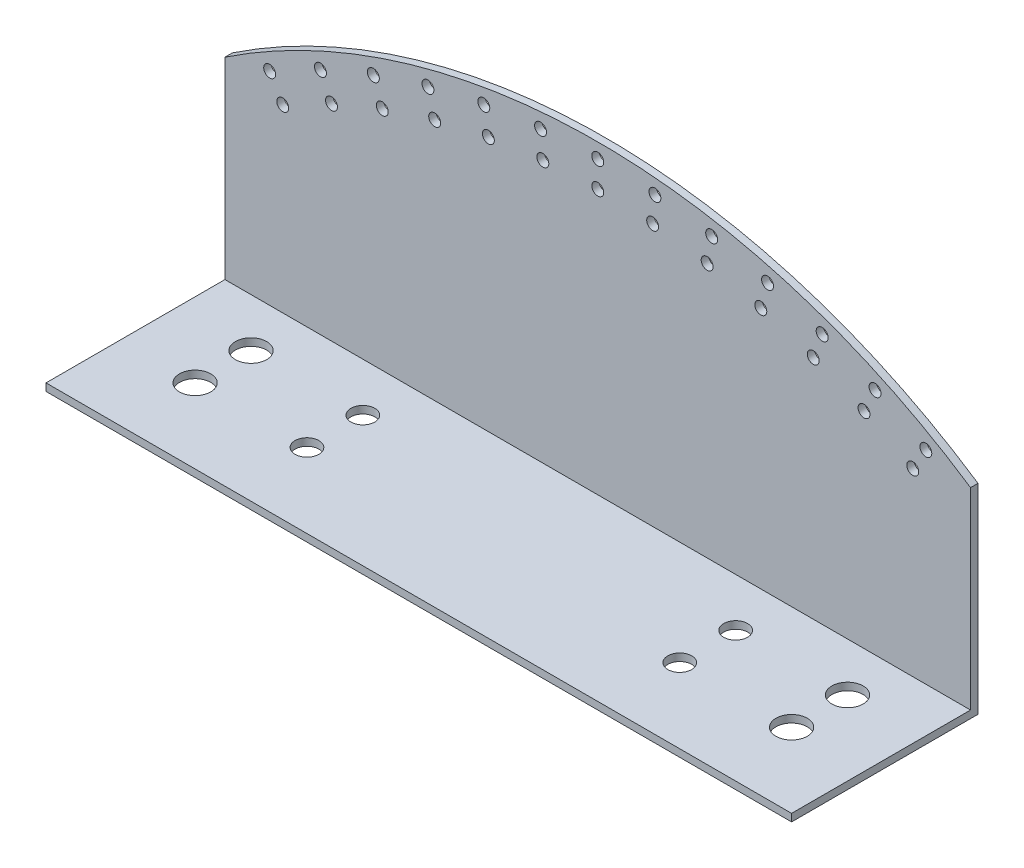
from build123d import *

# Parameters (mm, degrees)
SKETCH_1_R          = 1.6
EXTRUDE_1_DEPTH     = 2
SKETCH_2_W          = 200
SKETCH_2_H          = 2
EXTRUDE_2_DEPTH     = 48
SKETCH_3_R          = 3.2
SKETCH_3_R_2        = 4.2
CUT_EXTRUDE_1_DEPTH = 48


with BuildPart() as part:
    # 草图1 → 凸台-拉伸1 (new body)
    with BuildSketch(Plane.XY):
        with BuildLine():
            Line((1437.273715593, 307.480108419), (1237.273715593, 307.480108419))
            Line((1237.273715593, 307.480108419), (1237.273715593, 361.14640389))
            ThreePointArc((1237.273715593, 361.14640389), (1337.273715593, 391.480108419), (1437.273715593, 361.14640389))
            Line((1437.273715593, 361.14640389), (1437.273715593, 307.480108419))
        make_face()
        with Locations((1337.273715593, 387.480108419)):
            Circle(SKETCH_1_R, mode=Mode.SUBTRACT)
        with Locations((1337.273715593, 380.480108419)):
            Circle(SKETCH_1_R, mode=Mode.SUBTRACT)
        with Locations((1321.934304869, 386.810375283)):
            Circle(SKETCH_1_R, mode=Mode.SUBTRACT)
        with Locations((1322.544395068, 379.837012397)):
            Circle(SKETCH_1_R, mode=Mode.SUBTRACT)
        with Locations((1306.711636323, 384.806272949)):
            Circle(SKETCH_1_R, mode=Mode.SUBTRACT)
        with Locations((1307.927173567, 377.912618678)):
            Circle(SKETCH_1_R, mode=Mode.SUBTRACT)
        with Locations((1291.721563655, 381.483053846)):
            Circle(SKETCH_1_R, mode=Mode.SUBTRACT)
        with Locations((1293.53329697, 374.721573062)):
            Circle(SKETCH_1_R, mode=Mode.SUBTRACT)
        with Locations((1277.078170367, 376.866009678)):
            Circle(SKETCH_1_R, mode=Mode.SUBTRACT)
        with Locations((1279.472311371, 370.288161332)):
            Circle(SKETCH_1_R, mode=Mode.SUBTRACT)
        with Locations((1262.892901526, 370.990278938)):
            Circle(SKETCH_1_R, mode=Mode.SUBTRACT)
        with Locations((1265.851229359, 364.646124428)):
            Circle(SKETCH_1_R, mode=Mode.SUBTRACT)
        with Locations((1249.273715593, 363.900579485)):
            Circle(SKETCH_1_R, mode=Mode.SUBTRACT)
        with Locations((1252.773715593, 357.838401659)):
            Circle(SKETCH_1_R, mode=Mode.SUBTRACT)
        with Locations((1425.273715593, 363.900579485)):
            Circle(SKETCH_1_R, mode=Mode.SUBTRACT)
        with Locations((1421.773715593, 357.838401659)):
            Circle(SKETCH_1_R, mode=Mode.SUBTRACT)
        with Locations((1411.654529659, 370.990278938)):
            Circle(SKETCH_1_R, mode=Mode.SUBTRACT)
        with Locations((1408.696201827, 364.646124428)):
            Circle(SKETCH_1_R, mode=Mode.SUBTRACT)
        with Locations((1397.469260818, 376.866009678)):
            Circle(SKETCH_1_R, mode=Mode.SUBTRACT)
        with Locations((1395.075119815, 370.288161332)):
            Circle(SKETCH_1_R, mode=Mode.SUBTRACT)
        with Locations((1382.825867531, 381.483053846)):
            Circle(SKETCH_1_R, mode=Mode.SUBTRACT)
        with Locations((1381.014134215, 374.721573062)):
            Circle(SKETCH_1_R, mode=Mode.SUBTRACT)
        with Locations((1367.835794862, 384.806272949)):
            Circle(SKETCH_1_R, mode=Mode.SUBTRACT)
        with Locations((1366.620257618, 377.912618678)):
            Circle(SKETCH_1_R, mode=Mode.SUBTRACT)
        with Locations((1352.613126316, 386.810375283)):
            Circle(SKETCH_1_R, mode=Mode.SUBTRACT)
        with Locations((1352.003036117, 379.837012397)):
            Circle(SKETCH_1_R, mode=Mode.SUBTRACT)
    extrude(amount=EXTRUDE_1_DEPTH)

    # 草图2 → 凸台-拉伸2 (add)
    with BuildSketch(Plane.XY.offset(2)):
        with Locations((1337.273715593, 308.480108419)):
            Rectangle(SKETCH_2_W, SKETCH_2_H)
    extrude(amount=EXTRUDE_2_DEPTH)

    # 草图3 → 切除-拉伸1 (cut)
    with BuildSketch(Plane(origin=(0, 309.480108419, 0), x_dir=(1, 0, 0), z_dir=(0, 1, 0))):
        with Locations(Location((1287.273715593, -30, 0), (0, 0, 270))):
            Circle(SKETCH_3_R)
        with Locations(Location((1387.273715593, -30, 0), (0, 0, 270))):
            Circle(SKETCH_3_R)
        with Locations(Location((1257.273715593, -15, 0), (0, 0, 270))):
            Circle(SKETCH_3_R_2)
        with Locations(Location((1417.273715593, -15, 0), (0, 0, 270))):
            Circle(SKETCH_3_R_2)
        with Locations(Location((1257.273715593, -30, 0), (0, 0, 270))):
            Circle(SKETCH_3_R_2)
        with Locations(Location((1287.273715593, -15, 0), (0, 0, 270))):
            Circle(SKETCH_3_R)
        with Locations(Location((1387.273715593, -15, 0), (0, 0, 270))):
            Circle(SKETCH_3_R)
        with Locations(Location((1417.273715593, -30, 0), (0, 0, 270))):
            Circle(SKETCH_3_R_2)
    extrude(amount=-CUT_EXTRUDE_1_DEPTH, mode=Mode.SUBTRACT)


solid = part.part
